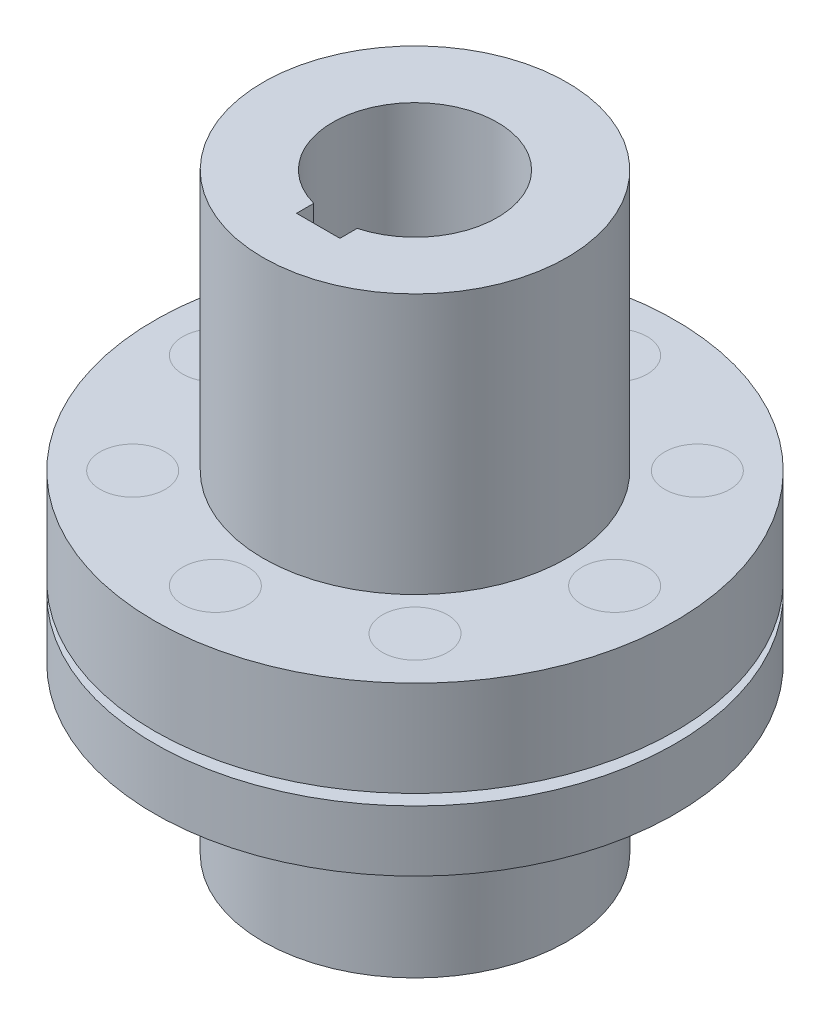
SolidWorks part; units mm, degrees
ref_plane "Front Plane" through (0, 0, 0) normal (0, 0, 1) x (1, 0, 0)
ref_plane "Top Plane" through (0, 0, 0) normal (0, 1, 0) x (1, 0, 0)
ref_plane "Right Plane" through (0, 0, 0) normal (1, 0, 0) x (0, 0, -1)
sketch "Sketch 1" plane through (0, 0, 0) normal (0, 0, 1) x (1, 0, 0)
  line L0 (0, 116.5729) -> (0, -54.0313) construction
  line L1 (-90.6458, 0) -> (93.0208, 0) construction
  line L2 (-19, 15) -> (-19, 82)
  line L3 (-19, 82) -> (-35, 82)
  line L4 (-35, 82) -> (-35, 22)
  line L5 (-35, 22) -> (-60, 22)
  line L6 (-60, 22) -> (-60, 0)
  line L7 (-60, 0) -> (-24, 0)
  line L8 (-19, 15) -> (-24, 15)
  line L9 (-24, 15) -> (-24, 0)
  dimension "D1" = 38
  dimension "D2" = 120
  dimension "D3" = 60
  dimension "D4" = 82
  dimension "D5" = 70
  dimension "D6" = 5
  dimension "D7" = 15
revolve "Revolve 1" add sketch "Sketch 1" angle 360 about L0
sketch "Sketch 2" plane through (0, 22, 0) normal (0, 1, 0) x (1, 0, 0)
  circle A0 centre (0, 0) radius 46 construction
  circle A1 centre (0, -46) radius 7.5
  circle A2 centre (-32.5269, -32.5269) radius 7.5
  circle A3 centre (-46, 0) radius 7.5
  circle A4 centre (-32.5269, 32.5269) radius 7.5
  circle A5 centre (0, 46) radius 7.5
  circle A6 centre (32.5269, 32.5269) radius 7.5
  circle A7 centre (46, 0) radius 7.5
  circle A8 centre (32.5269, -32.5269) radius 7.5
  point P21 (0, 0)
  dimension "D1" = 15
  dimension "D2" = 92
  dimension "D3" = 8
extrude "Cut-Extrude 1" cut sketch "Sketch 2" against normal through all
sketch "Sketch 3" plane through (0, 22, 0) normal (0, 1, 0) x (1, 0, 0)
  circle A0 centre (0, -46) radius 7.5 construction
  circle A1 centre (0, -46) radius 7.5
  circle A2 centre (-32.5269, -32.5269) radius 7.5
  circle A3 centre (-46, 0) radius 7.5
  circle A4 centre (-32.5269, 32.5269) radius 7.5
  circle A5 centre (0, 46) radius 7.5
  circle A6 centre (32.5269, 32.5269) radius 7.5
  circle A7 centre (46, 0) radius 7.5
  circle A8 centre (32.5269, -32.5269) radius 7.5
  point P19 (0, 0)
  dimension "D1" = 8
extrude "Boss-Extrude 1" add sketch "Sketch 3" against normal blind 38.5 separate body
sketch "Sketch 4" plane through (0, 0, 0) normal (0, -1, 0) x (1, 0, 0)
  circle A0 centre (-32.5269, 32.5269) radius 7.5 construction
  circle A1 centre (0, 0) radius 60
  circle A2 centre (0, 0) radius 60
  circle A3 centre (-46, 0) radius 7.5 construction
  circle A4 centre (-32.5269, -32.5269) radius 7.5 construction
  circle A5 centre (0, -46) radius 7.5 construction
  circle A6 centre (32.5269, -32.5269) radius 7.5 construction
  circle A7 centre (46, 0) radius 7.5 construction
  circle A8 centre (32.5269, 32.5269) radius 7.5 construction
  circle A9 centre (0, 46) radius 7.5 construction
  circle A10 centre (-32.5269, 32.5269) radius 7.5
  circle A11 centre (-46, 0) radius 7.5
  circle A12 centre (-32.5269, -32.5269) radius 7.5
  circle A13 centre (0, -46) radius 7.5
  circle A14 centre (32.5269, -32.5269) radius 7.5
  circle A15 centre (46, 0) radius 7.5
  circle A16 centre (32.5269, 32.5269) radius 7.5
  circle A17 centre (0, 46) radius 7.5
  circle A18 centre (0, 0) radius 10
  dimension "D2" = 20
  dimension "D1" = 0
extrude "Boss-Extrude 2" add sketch "Sketch 4" along normal blind 14 from offset 2.5 separate body
sketch "Sketch 5" plane through (0, -16.5, 0) normal (0, -1, 0) x (1, 0, 0)
  circle A0 centre (0, 0) radius 10 construction
  circle A1 centre (0, 0) radius 10
  circle A2 centre (0, 0) radius 35
  dimension "D1" = 70
extrude "Boss-Extrude 3" add sketch "Sketch 5" along normal blind 38
sketch "Sketch 6" plane through (0, -54.5, 0) normal (0, -1, 0) x (1, 0, 0)
  line L0 (0, 70.0558) -> (0, -33.47) construction
  line L1 (-3, 9.5394) -> (-3, 12.8)
  line L2 (-3, 12.8) -> (3, 12.8)
  line L3 (3, 9.5394) -> (3, 12.8)
  circle A0 centre (0, 0) radius 10 construction
  arc A1 (3, 9.5394) -> (-3, 9.5394) centre (0, 0) ccw
  point P6 (0, 10)
  point P10 (0, 12.8)
  dimension "D1" = 6
  dimension "D2" = 2.8
extrude "Cut-Extrude 2" cut sketch "Sketch 6" against normal up to surface (52 mm away) up to face at (0, -2.5, -60)
sketch "Sketch 7" plane through (0, 82, 0) normal (0, 1, 0) x (1, 0, 0)
  line L0 (0, -65.975) -> (0, 29.5501) construction
  line L1 (5, -18.3303) -> (5, -22.3)
  line L2 (5, -22.3) -> (-5, -22.3)
  line L3 (-5, -18.3303) -> (-5, -22.3)
  circle A0 centre (0, 0) radius 19 construction
  arc A1 (-5, -18.3303) -> (5, -18.3303) centre (0, 0) ccw
  point P9 (0, -19)
  point P10 (0, -22.3)
  dimension "D1" = 10
  dimension "D2" = 3.3
extrude "Cut-Extrude 3" cut sketch "Sketch 7" against normal up to next (67 mm away)
